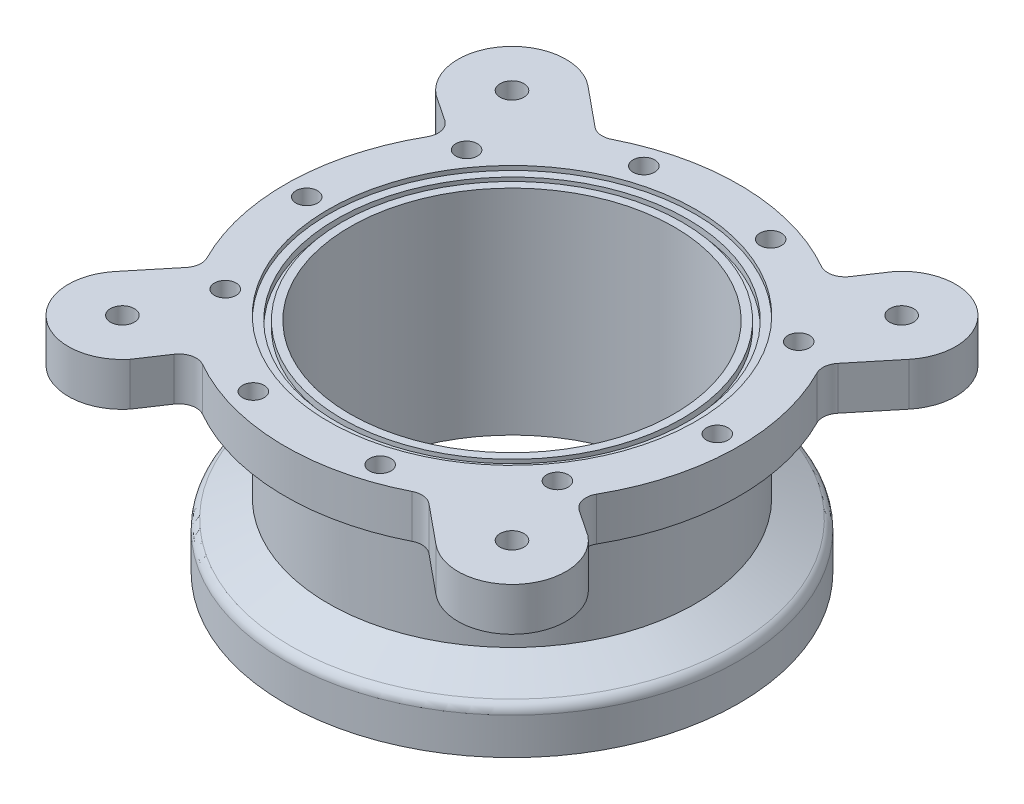
from build123d import *

# Parameters (mm, degrees)
SKETCH_2_OUTSIDE_W       = 395.692
SKETCH_2_OUTSIDE_H       = 395.692
CUT_EXTRUDE_1_DEPTH      = 43
SKETCH_2_3_R             = 5.5
SKETCH_2_3_R_2           = 4
CUT_EXTRUDE_2_DEPTH      = 43
SKETCH_3_R               = 5
CUT_EXTRUDE_4_DEPTH      = 16
PATTERN_CIRCULAR_2_COUNT = 10
SKETCH_22_R              = 11
CUT_EXTRUDE_13_DEPTH     = 2.6
CUT_EXTRUDE_17_DEPTH     = 47.2


with BuildPart() as part:
    # 草图1 → 旋转1 (revolve)
    with BuildSketch(Plane(origin=(0, 0, 0), x_dir=(0, 0, -1), z_dir=(1, 0, 0))):
        with BuildLine():
            Line((85, 98), (85, 55))
            Line((85, 55), (102.2172823, 46.481479577))
            ThreePointArc((102.2172823, 46.481479577), (104.247729482, 44.637573553), (105, 42))
            Line((105, 42), (105, 25))
            Line((105, 25), (85, 25))
            Line((85, 25), (85, 27))
            Line((85, 27), (81.25, 27))
            Line((81.25, 27), (81.25, 30))
            Line((81.25, 30), (78.75, 30))
            Line((78.75, 30), (78.75, 27))
            Line((78.75, 27), (75, 27))
            Line((75, 27), (75, 126))
            Line((75, 126), (78.75, 126))
            Line((78.75, 126), (78.75, 123))
            Line((78.75, 123), (80, 123))
            Line((80, 123), (81.25, 123))
            Line((81.25, 123), (81.25, 126))
            Line((81.25, 126), (85, 126))
            Line((85, 126), (85, 128))
            Line((85, 128), (152.5, 128))
            Line((152.5, 128), (152.5, 108))
            Line((152.5, 108), (105, 108))
            Line((105, 108), (85, 98))
        make_face()
    revolve(axis=Axis((0, 0, 0), (0, 1, 0)))

    # 草图2 outside → 切除-拉伸1 (cut)
    with BuildSketch(Plane(origin=(0, 128, 0), x_dir=(1, 0, 0), z_dir=(0, 1, 0))):
        Rectangle(SKETCH_2_OUTSIDE_W, SKETCH_2_OUTSIDE_H)
        with BuildLine():
            Line((106.015518025, -70.830501466), (93.723088078, -62.617751167))
            ThreePointArc((93.723088078, -62.617751167), (90.381359185, -57.803804637), (91.217453609, -52.003616769))
            ThreePointArc((91.217453609, -52.003616769), (96.412361456, -41.589139911), (100.422788605, -30.663716814))
            ThreePointArc((100.422788605, -30.663716814), (103.31433575, -26.569981902), (108.074048689, -25))
            Line((108.074048689, -25), (127.5, -25))
            ThreePointArc((127.5, -25), (152.5, 0), (127.5, 25))
            Line((127.5, 25), (108.074048689, 25))
            ThreePointArc((108.074048689, 25), (103.31433575, 26.569981902), (100.422788605, 30.663716814))
            ThreePointArc((100.422788605, 30.663716814), (97.401647161, 39.216312045), (93.653644879, 47.476255126))
            ThreePointArc((93.653644879, 47.476255126), (92.836646991, 51.963853326), (94.604964476, 56.168502708))
            Line((94.604964476, 56.168502708), (109.481727736, 74.296711178))
            ThreePointArc((109.481727736, 74.296711178), (106.015518025, 109.481727736), (70.830501466, 106.015518025))
            Line((70.830501466, 106.015518025), (62.617751167, 93.723088078))
            ThreePointArc((62.617751167, 93.723088078), (57.803804637, 90.381359185), (52.003616769, 91.217453609))
            ThreePointArc((52.003616769, 91.217453609), (2.570604567, 104.96852858), (-47.476255126, 93.653644879))
            ThreePointArc((-47.476255126, 93.653644879), (-51.963853326, 92.836646991), (-56.168502708, 94.604964476))
            Line((-56.168502708, 94.604964476), (-74.296711178, 109.481727736))
            ThreePointArc((-74.296711178, 109.481727736), (-109.481727736, 106.015518025), (-106.015518025, 70.830501466))
            Line((-106.015518025, 70.830501466), (-93.723088078, 62.617751167))
            ThreePointArc((-93.723088078, 62.617751167), (-90.381359185, 57.803804637), (-91.217453609, 52.003616769))
            ThreePointArc((-91.217453609, 52.003616769), (-96.412361456, 41.589139911), (-100.422788605, 30.663716814))
            ThreePointArc((-100.422788605, 30.663716814), (-103.31433575, 26.569981902), (-108.074048689, 25))
            Line((-108.074048689, 25), (-127.5, 25))
            ThreePointArc((-127.5, 25), (-152.5, 0), (-127.5, -25))
            Line((-127.5, -25), (-108.074048689, -25))
            ThreePointArc((-108.074048689, -25), (-103.31433575, -26.569981902), (-100.422788605, -30.663716814))
            ThreePointArc((-100.422788605, -30.663716814), (-97.401647161, -39.216312045), (-93.653644879, -47.476255126))
            ThreePointArc((-93.653644879, -47.476255126), (-92.836646991, -51.963853326), (-94.604964476, -56.168502708))
            Line((-94.604964476, -56.168502708), (-109.481727736, -74.296711178))
            ThreePointArc((-109.481727736, -74.296711178), (-106.015518025, -109.481727736), (-70.830501466, -106.015518025))
            Line((-70.830501466, -106.015518025), (-62.617751167, -93.723088078))
            ThreePointArc((-62.617751167, -93.723088078), (-57.803804637, -90.381359185), (-52.003616769, -91.217453609))
            ThreePointArc((-52.003616769, -91.217453609), (-2.570604567, -104.96852858), (47.476255126, -93.653644879))
            ThreePointArc((47.476255126, -93.653644879), (51.963853326, -92.836646991), (56.168502708, -94.604964476))
            Line((56.168502708, -94.604964476), (74.296711178, -109.481727736))
            ThreePointArc((74.296711178, -109.481727736), (109.481727736, -106.015518025), (106.015518025, -70.830501466))
        make_face(mode=Mode.SUBTRACT)
    extrude(amount=-CUT_EXTRUDE_1_DEPTH, mode=Mode.SUBTRACT)

    # 草图2<3> → 切除-拉伸2 (cut)
    with BuildSketch(Plane(origin=(0, 128, 0), x_dir=(1, 0, 0), z_dir=(0, 1, 0))):
        with Locations(Location((90.156114601, -90.156114601, 0), (0, 0, 270))):
            Circle(SKETCH_2_3_R)
        with Locations(Location((-90.156114601, -90.156114601, 0), (0, 0, 270))):
            Circle(SKETCH_2_3_R)
        with Locations(Location((-90.156114601, 90.156114601, 0), (0, 0, 270))):
            Circle(SKETCH_2_3_R)
        with Locations(Location((90.156114601, 90.156114601, 0), (0, 0, 270))):
            Circle(SKETCH_2_3_R)
        with Locations(Location((-127.5, 0, 0), (0, 0, 270))):
            Circle(SKETCH_2_3_R_2)
        with Locations(Location((127.5, 0, 0), (0, 0, 270))):
            Circle(SKETCH_2_3_R_2)
    extrude(amount=-CUT_EXTRUDE_2_DEPTH, mode=Mode.SUBTRACT)

    # 草图3 → 切除-拉伸4 (cut)
    with BuildSketch(Plane(origin=(0, 128, 0), x_dir=(1, 0, 0), z_dir=(0, 1, 0))):
        with Locations(Location((-95, 0, 0), (0, 0, 270))):
            Circle(SKETCH_3_R)
    cut_extrude_4 = extrude(amount=-CUT_EXTRUDE_4_DEPTH, mode=Mode.SUBTRACT)

    # 阵列(圆周)2: 切除-拉伸4 ×10 about axis
    pattern_circular_2_axis = Axis((0, 0, 0), (0, 1, 0))
    for i in range(1, PATTERN_CIRCULAR_2_COUNT):
        add(cut_extrude_4.rotate(pattern_circular_2_axis, i * 360 / PATTERN_CIRCULAR_2_COUNT), mode=Mode.SUBTRACT)

    # 草图22 → 切除-拉伸13 (cut)
    with BuildSketch(Plane.XZ.offset(-108)):
        with Locations(Location((90.156114601, -90.156114601, 0), (0, 0, 270))):
            Circle(SKETCH_22_R)
    extrude(amount=-CUT_EXTRUDE_13_DEPTH, mode=Mode.SUBTRACT)

    # 草图24 → 切除-拉伸17 (cut)
    with BuildSketch(Plane(origin=(0, 128, 0), x_dir=(1, 0, 0), z_dir=(0, 1, 0))):
        with BuildLine():
            Line((-100.422788605, 30.663716814), (-181.652372804, 37.940541355))
            Line((-181.652372804, 37.940541355), (-167.948313734, -59.042030524))
            Line((-167.948313734, -59.042030524), (-95.973272696, -42.592615887))
            ThreePointArc((-95.973272696, -42.592615887), (-104.806849937, -6.365862568), (-100.422788605, 30.663716814))
        make_face()
        with BuildLine():
            Line((97.905644994, 37.940541355), (167.274054284, 34.075293925))
            Line((167.274054284, 34.075293925), (170.436529454, -59.042030524))
            Line((170.436529454, -59.042030524), (95.973272696, -42.592615887))
            ThreePointArc((95.973272696, -42.592615887), (104.969786296, -2.518722898), (97.905644994, 37.940541355))
        make_face()
    extrude(amount=-CUT_EXTRUDE_17_DEPTH, mode=Mode.SUBTRACT)


solid = part.part
